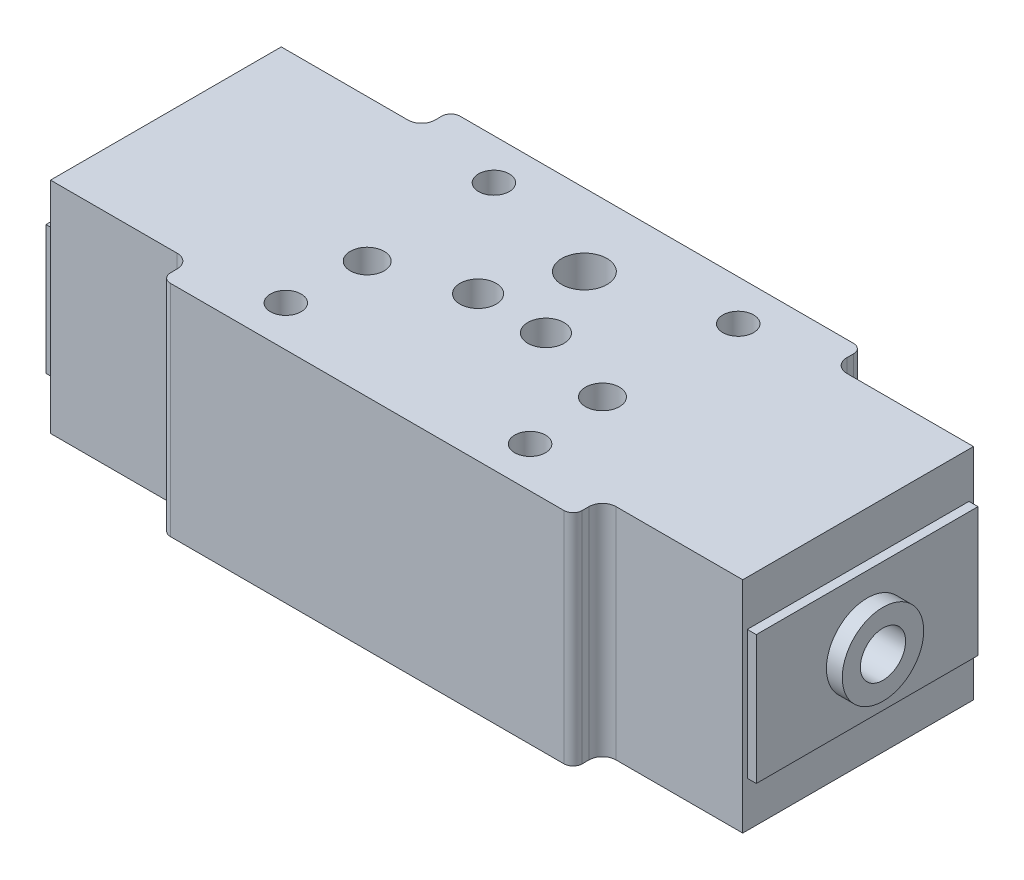
SolidWorks part; units mm, degrees
ref_plane "Front Plane" through (0, 0, 0) normal (0, 0, 1) x (1, 0, 0)
ref_plane "Top Plane" through (0, 0, 0) normal (0, 1, 0) x (1, 0, 0)
ref_plane "Right Plane" through (0, 0, 0) normal (1, 0, 0) x (0, 0, -1)
sketch "Sketch 1" plane through (0, 0, 0) normal (0, 1, 0) x (1, 0, 0)
  line L0 (0, 77.5231) -> (0, -81.4796) construction
  line L1 (-141.6929, 0) -> (168.1522, 0) construction
  line L2 (43.5, 32) -> (-43.5, 32)
  line L3 (-45.5, 30) -> (-45.5, 28.5)
  line L4 (-48.5, 25.5) -> (-76.5, 25.5)
  line L5 (-76.5, 25.5) -> (-76.5, -25.5)
  line L6 (-48.5, -25.5) -> (-76.5, -25.5)
  line L7 (-45.5, -30) -> (-45.5, -28.5)
  line L8 (43.5, -32) -> (-43.5, -32)
  line L9 (45.5, -30) -> (45.5, -28.5)
  line L10 (48.5, -25.5) -> (76.5, -25.5)
  line L11 (76.5, 25.5) -> (76.5, -25.5)
  line L12 (48.5, 25.5) -> (76.5, 25.5)
  line L13 (45.5, 30) -> (45.5, 28.5)
  arc A0 (-43.5, 32) -> (-45.5, 30) centre (-43.5, 30) ccw
  arc A1 (-45.5, 28.5) -> (-48.5, 25.5) centre (-48.5, 28.5) cw
  arc A2 (-45.5, -28.5) -> (-48.5, -25.5) centre (-48.5, -28.5) ccw
  arc A3 (-43.5, -32) -> (-45.5, -30) centre (-43.5, -30) cw
  arc A4 (43.5, -32) -> (45.5, -30) centre (43.5, -30) ccw
  arc A5 (45.5, -28.5) -> (48.5, -25.5) centre (48.5, -28.5) cw
  arc A6 (45.5, 28.5) -> (48.5, 25.5) centre (48.5, 28.5) ccw
  arc A7 (43.5, 32) -> (45.5, 30) centre (43.5, 30) cw
  point P5 (76.5, 0)
  point P21 (-76.5, 0)
  point P34 (0, -32)
  point P36 (0, 32)
  dimension "D5" = 2
  dimension "D6" = 3
  dimension "D1" = 91
  dimension "D2" = 51
  dimension "D3" = 6.5
  dimension "D4" = 153
extrude "Boss-Extrude 1" add sketch "Sketch 1" along normal mid plane 48.5
sketch "Sketch 2" plane through (76.5, 0, 0) normal (1, 0, 0) x (0, 0, -1)
  line L0 (0, 29.9912) -> (0, -30.5638) construction
  line L1 (-35.6459, 0) -> (39.7974, 0) construction
  line L2 (-25.5, 24.25) -> (25.5, 24.25) construction
  line L3 (-24.5, -14.25) -> (24.5, -14.25)
  line L4 (-24.5, -14.25) -> (-24.5, 14.25)
  line L5 (-24.5, 14.25) -> (24.5, 14.25)
  line L6 (24.5, -14.25) -> (24.5, 14.25)
  line L7 (-24.5, -14.25) -> (24.5, 14.25) construction
  line L8 (-24.5, 14.25) -> (24.5, -14.25) construction
  line L9 (-25.5, 24.25) -> (-25.5, -24.25) construction
  circle A0 centre (0, 0) radius 3.0243
  point P5 (0, 0)
  dimension "D1" = 10
  dimension "D2" = 1
extrude "Boss-Extrude 2" add sketch "Sketch 2" along normal blind 2
sketch "Sketch 3" plane through (76.5, 0, 0) normal (1, 0, 0) x (0, 0, -1)
  circle A0 centre (0, 0) radius 9
  dimension "D1" = 18
extrude "Boss-Extrude 3" add sketch "Sketch 3" along normal blind 5.5
mirror "Mirror 1" about plane through (0, 0, 0) normal (1, 0, 0) of "Boss-Extrude 3", "Boss-Extrude 2"
sketch "Sketch 4" plane through (0, 24.25, 0) normal (0, 1, 0) x (1, 0, 0)
  line L0 (0, 37.8938) -> (0, -46.1731) construction
  line L1 (-91.9216, 0) -> (90.8602, 0) construction
  line L2 (-76.5, 25.5) -> (-76.5, -25.5) construction
  circle A0 centre (-27, 23) radius 3.4
  circle A1 centre (0, 16) radius 5
  circle A2 centre (-7.5, 0) radius 4
  circle A3 centre (-26, -6) radius 3.75
  circle A4 centre (-27, -23) radius 3.4
  circle A5 centre (7.5, 0) radius 4
  circle A6 centre (27, -23) radius 3.4
  circle A7 centre (26, -6) radius 3.75
  circle A8 centre (27, 23) radius 3.4
  dimension "D1" = 6.8
  dimension "D2" = 49.5
  dimension "D3" = 46
  dimension "D4" = 10
  dimension "D5" = 16
  dimension "D6" = 8
  dimension "D7" = 15
  dimension "D8" = 7.5
  dimension "D9" = 52
  dimension "D10" = 12
extrude "Cut-Extrude 1" cut sketch "Sketch 4" against normal through all
sketch "Sketch 5" plane through (82, 0, 0) normal (1, 0, 0) x (0, 0, -1)
  circle A0 centre (0, 0) radius 5
  dimension "D1" = 10
extrude "Cut-Extrude 2" cut sketch "Sketch 5" against normal through all
